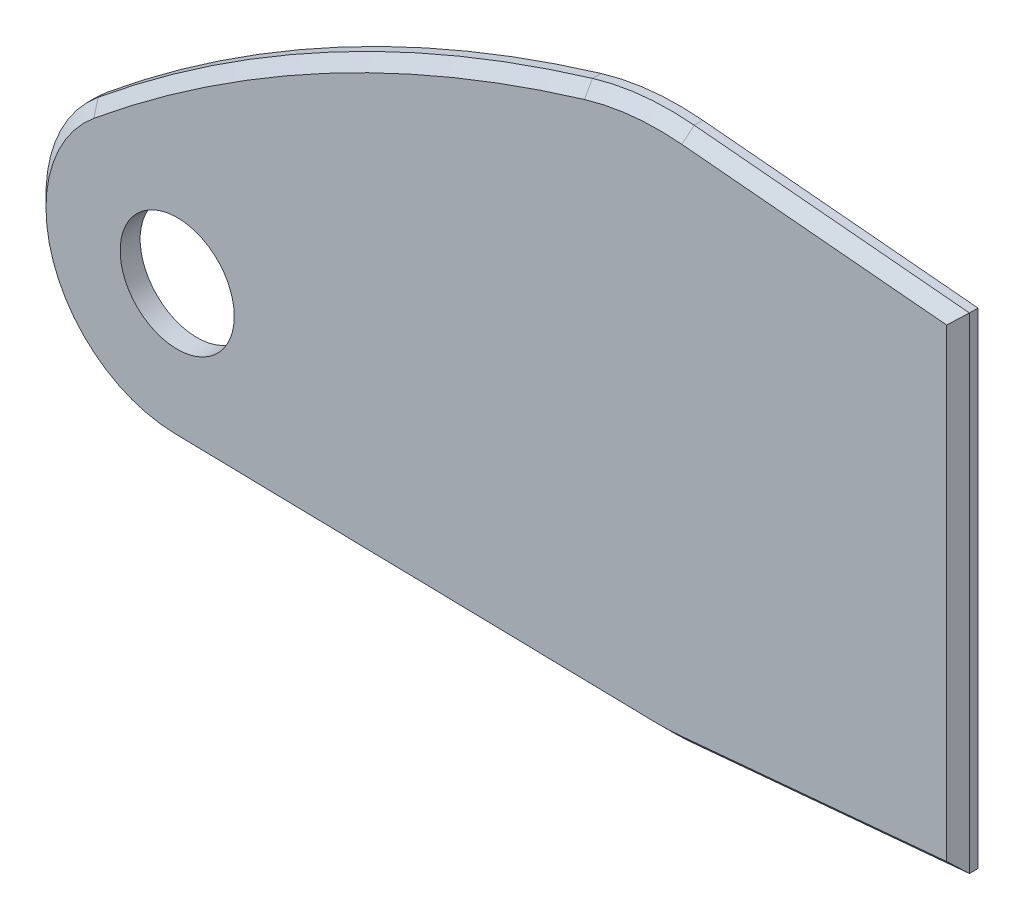
SolidWorks part; units mm, degrees
ref_plane "Front Plane" through (0, 0, 0) normal (0, 0, 1) x (1, 0, 0)
ref_plane "Top Plane" through (0, 0, 0) normal (0, 1, 0) x (1, 0, 0)
ref_plane "Right Plane" through (0, 0, 0) normal (1, 0, 0) x (0, 0, -1)
sketch "Sketch1" plane through (0, 0, 0) normal (0, 0, 1) x (1, 0, 0)
  line L0 (-124.7492, 0) -> (162.3726, 0) construction
  line L1 (0, 225.6352) -> (0, -123.7667) construction
  line L2 (210, 170.2) -> (17.0529, 187.7271)
  line L3 (-339.5495, -181.579) -> (-3.8634, -188.4604)
  line L4 (210, -170.2) -> (17.0529, -187.7271)
  line L5 (210, 170.2) -> (210, -170.2)
  circle A0 centre (-337.5, -81.6) radius 40
  arc A1 (-400.9638, -4.3191) -> (-339.5495, -181.579) centre (-337.5, -81.6) ccw
  arc A2 (17.0529, 187.7271) -> (-54.2793, 180.516) centre (0, 0) ccw
  arc A3 (-54.2793, 180.516) -> (-400.9638, -4.3191) centre (233.6745, -777.1284) ccw
  arc A4 (-3.8634, -188.4604) -> (17.0529, -187.7271) centre (0, 0) ccw
  dimension "D3" = 80
  dimension "D4" = 200
  dimension "D6" = 377
  dimension "D7" = 2000
  dimension "D1" = 81.6
  dimension "D2" = 337.5
  dimension "D5" = 210
  dimension "D9" = 170.2
  dimension "D10" = 170.2
extrude "Boss-Extrude1" add sketch "Sketch1" along normal blind 14
chamfer "Chamfer1" distance 8 angle 45 8 edges at (-18.9592, 187.5441, 14) (-236.7881, 105.2916, 14) (-431.9895, -114.3373, 14) (-171.7064, -185.0197, 14) (6.6049, -188.3842, 14) (113.5264, -178.9635, 14) (210, 0, 14) (113.5264, 178.9635, 14)
